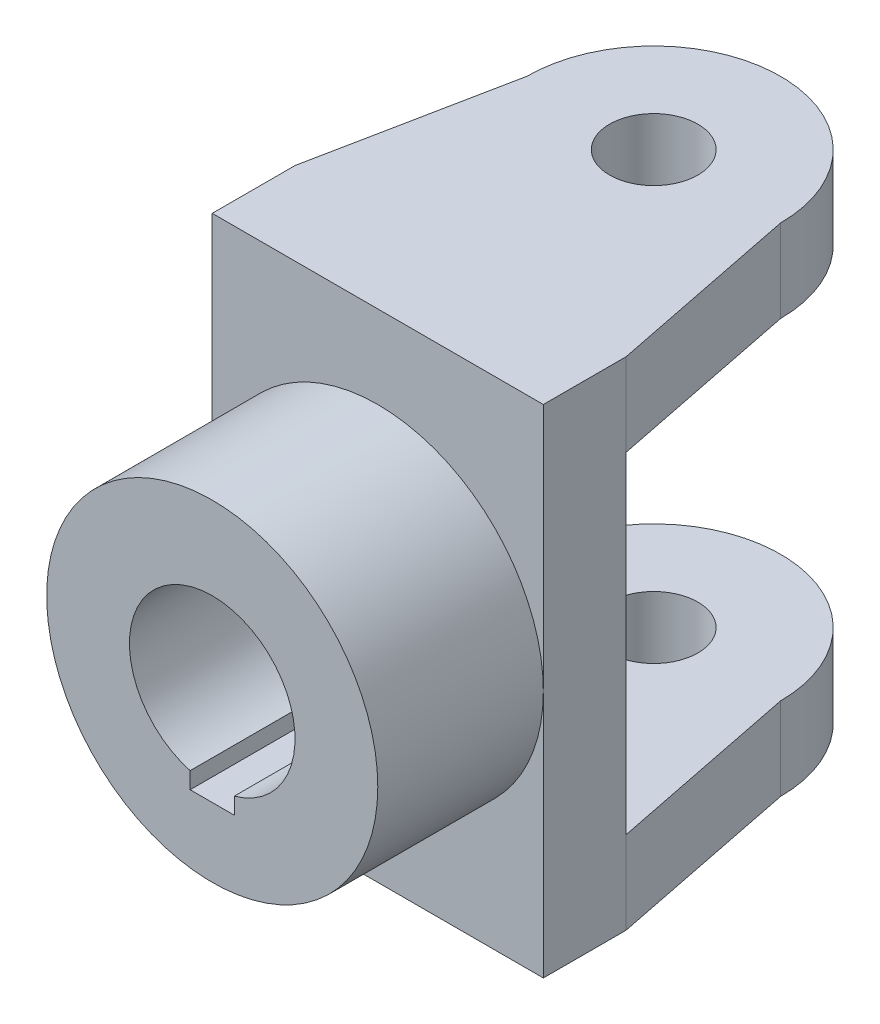
SolidWorks part; units mm, degrees
ref_plane "Front Plane" through (0, 0, 0) normal (0, 0, 1) x (1, 0, 0)
ref_plane "Top Plane" through (0, 0, 0) normal (0, 1, 0) x (1, 0, 0)
ref_plane "Right Plane" through (0, 0, 0) normal (1, 0, 0) x (0, 0, -1)
sketch "Sketch1" plane through (0, 0, 0) normal (0, 0, 1) x (1, 0, 0)
  line L1 (-30, 45) -> (30, 45)
  line L2 (-30, 45) -> (-30, -45)
  line L3 (-30, -45) -> (30, -45)
  line L4 (30, 45) -> (30, -45)
  line L5 (-30, 45) -> (30, -45) construction
  line L6 (-30, -45) -> (30, 45) construction
  point P0 (0, 0)
  dimension "D1" = 90
  dimension "D2" = 60
extrude "Boss-Extrude1" add sketch "Sketch1" against normal blind 15
ref_plane "Plane1" through (0, 45, 0) normal (0, 1, 0) x (1, 0, 0)
sketch "Sketch2" plane through (0, 45, 0) normal (0, 1, 0) x (1, 0, 0)
  line L0 (-23, 50) -> (-30, 15)
  line L1 (30, 15) -> (-30, 15) construction
  line L2 (-30, 15) -> (-30, 0) construction
  line L3 (30, 15) -> (23, 50)
  line L4 (-30, 15) -> (30, 15)
  circle A0 centre (0, 50) radius 8
  arc A1 (23, 50) -> (-23, 50) centre (0, 50) ccw
  dimension "D2" = 46
  dimension "D3" = 16
  dimension "D1" = 35
extrude "Boss-Extrude2" add sketch "Sketch2" against normal blind 15 contours A1 L0 L4 L3
mirror "Mirror1" about plane through (0, 0, 0) normal (0, 1, 0) of "Boss-Extrude2"
sketch "Sketch3" plane through (0, 0, 0) normal (0, 0, 1) x (1, 0, 0)
  line L2 (-4, -14.4568) -> (-4, -17.4568)
  line L3 (-4, -17.4568) -> (4, -17.4568)
  line L4 (4, -14.4568) -> (4, -17.4568)
  circle A0 centre (0, 0) radius 30
  arc A1 (4, -14.4568) -> (-4, -14.4568) centre (0, 0) ccw
  point P8 (0, -17.4568)
  dimension "D1" = 60
  dimension "D2" = 30
  dimension "D3" = 8
  dimension "D4" = 3
extrude "Boss-Extrude3" add sketch "Sketch3" along normal blind 30
